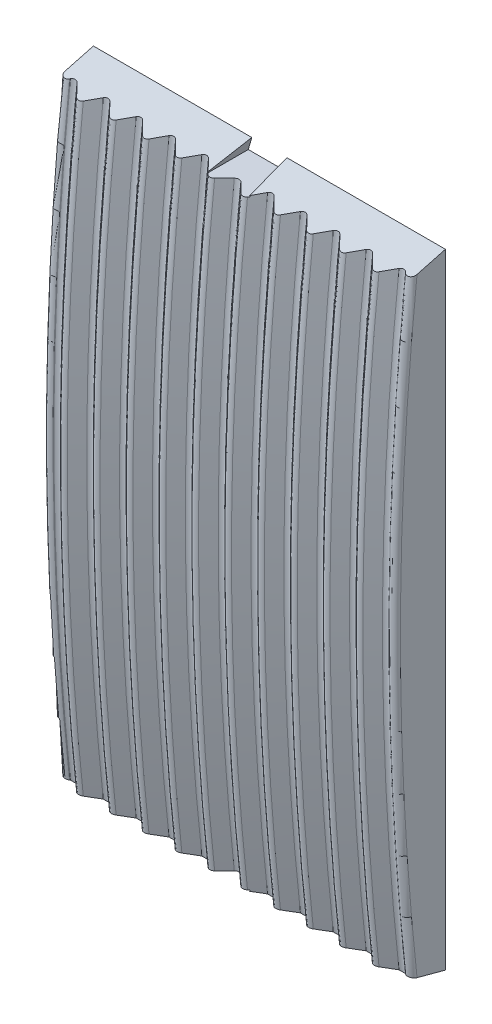
from build123d import *

# Parameters (mm, degrees)
BOSS_EXTRUDE1_DEPTH      = 375
CUT_EXTRUDE1_DEPTH       = 750
LPATTERN1_COUNT          = 6
LPATTERN1_PITCH          = 70
LPATTERN2_COUNT          = 6
LPATTERN2_PITCH          = 70
FILLET1_R                = 10
SKETCH6_W                = 315
SKETCH6_H                = 250
CUT_EXTRUDE2_DEPTH       = 60
CUT_EXTRUDE3_DEPTH       = 335
BOSS_EXTRUDE2_REACH      = 775.751
BOSS_EXTRUDE2_END_RADIUS = 5930
SKETCH8_W                = 40
SKETCH8_H                = 170
SKETCH8_W_2              = 35
SKETCH8_H_2              = 250


with BuildPart() as part:
    # Sketch2 → Boss-Extrude1 (new, symmetric)
    with BuildSketch(Plane(origin=(0, 0, 0), x_dir=(0, 0, -1), z_dir=(1, 0, 0))):
        with BuildLine():
            Line((130, -665), (130, 665))
            Line((130, 665), (34.157984961, 639.319209469))
            ThreePointArc((34.157984961, 639.319209469), (0, 0), (34.157984961, -639.319209469))
            Line((34.157984961, -639.319209469), (130, -665))
        make_face()
    extrude(amount=BOSS_EXTRUDE1_DEPTH, both=True)

    # Sketch3 → Cut-Extrude1 (cut)
    with BuildSketch(Plane(origin=(0, 0, -130), x_dir=(-1, 0, 0), z_dir=(0, 0, -1))):
        Polygon((-37.5, 665), (-45, 639), (45, 639), (37.5, 665), align=None)
    cut_extrude1 = extrude(amount=-CUT_EXTRUDE1_DEPTH, mode=Mode.SUBTRACT)

    # Mirror1: Cut-Extrude1 across plane
    add(cut_extrude1.mirror(Plane.ZX), mode=Mode.SUBTRACT)

    # Cut-Sweep1: sweep along a path in Sketch4
    with BuildLine(Plane(origin=(0, 0, 0), x_dir=(0, 0, -1), z_dir=(1, 0, 0))) as cut_sweep1_path:
        ThreePointArc((36.96595683, 665), (0, 0), (36.96595683, -665))
    # Sketch5 → Cut-Sweep1 (sweep, cut)
    with BuildSketch(Plane(origin=(0, 0, 0), x_dir=(1, 0, 0), z_dir=(0, 1, 0))):
        Polygon((0, 35), (-35, 0), (35, 0), align=None)
    cut_sweep1 = sweep(path=cut_sweep1_path.line, mode=Mode.SUBTRACT)

    # LPattern1: Cut-Sweep1 ×6
    with Locations(*[(-i * LPATTERN1_PITCH, 0, 0) for i in range(1, LPATTERN1_COUNT)]):
        add(cut_sweep1, mode=Mode.SUBTRACT)

    # LPattern2: Cut-Sweep1 ×6
    with Locations(*[(i * LPATTERN2_PITCH, 0, 0) for i in range(1, LPATTERN2_COUNT)]):
        add(cut_sweep1, mode=Mode.SUBTRACT)

    # Fillet1
    fillet1_edges = [part.edges().sort_by_distance(p)[0] for p in [
        (-350, 0, -35),
        (-375, 0, -10),
        (140, 0, -35),
        (210, 0, -35),
        (280, 0, -35),
        (350, 0, -35),
        (375, 0, -10),
        (315, 0, 0),
        (245, 0, 0),
        (175, 0, 0),
        (70, 0, -35),
        (0, 0, -35),
        (105, 0, 0),
        (35, 0, 0),
        (-35, 0, 0),
        (-70, 0, -35),
        (-105, 0, 0),
        (-140, 0, -35),
        (-175, 0, 0),
        (-210, 0, -35),
        (-245, 0, 0),
        (-280, 0, -35),
        (-315, 0, 0),
    ]]
    fillet(fillet1_edges, radius=FILLET1_R)

    # Sketch6 → Cut-Extrude2 (cut)
    with BuildSketch(Plane(origin=(0, 0, -130), x_dir=(-1, 0, 0), z_dir=(0, 0, -1))):
        with Locations((177.5, 0)):
            Rectangle(SKETCH6_W, SKETCH6_H)
        with Locations((-177.5, 0)):
            Rectangle(SKETCH6_W, SKETCH6_H)
    extrude(amount=-CUT_EXTRUDE2_DEPTH, mode=Mode.SUBTRACT)

    # Sketch7 → Cut-Extrude3 (cut, symmetric)
    with BuildSketch(Plane(origin=(0, 0, 0), x_dir=(0, 0, -1), z_dir=(1, 0, 0))):
        with BuildLine():
            Line((130, 625), (130, 455))
            Line((130, 455), (87.481501086, 455))
            ThreePointArc((87.481501086, 455), (94.643145913, 540.055947001), (103.028319552, 625))
            Line((103.028319552, 625), (130, 625))
        make_face()
        with BuildLine():
            Line((130, 415), (130, 165))
            Line((130, 165), (72.295975675, 165))
            ThreePointArc((72.295975675, 165), (77.098470758, 290.064604699), (84.539324786, 415))
            Line((84.539324786, 415), (130, 415))
        make_face()
    cut_extrude3 = extrude(amount=CUT_EXTRUDE3_DEPTH, both=True, mode=Mode.SUBTRACT)

    # Boss-Extrude2: up to this cylinder (the profile starts inside it)
    boss_extrude2_end = Plane(origin=(0, 0, -6000), z_dir=(1, 0, 0)) * Cylinder(BOSS_EXTRUDE2_END_RADIUS, 13647.502, mode=Mode.PRIVATE)
    # Sketch8 → Boss-Extrude2 (add, up to the surface)
    with BuildSketch(Plane(origin=(0, 0, -130), x_dir=(-1, 0, 0), z_dir=(0, 0, -1)), mode=Mode.PRIVATE) as boss_extrude2_sk1:
        with Locations((0, 540)):
            Rectangle(SKETCH8_W, SKETCH8_H)
    boss_extrude2_tool1 = extrude(boss_extrude2_sk1.sketch, amount=-BOSS_EXTRUDE2_REACH, mode=Mode.PRIVATE) & boss_extrude2_end
    # Sketch8 → Boss-Extrude2 (add, up to the surface)
    with BuildSketch(Plane(origin=(0, 0, -130), x_dir=(-1, 0, 0), z_dir=(0, 0, -1)), mode=Mode.PRIVATE) as boss_extrude2_sk2:
        with Locations((-117.5, 290)):
            Rectangle(SKETCH8_W_2, SKETCH8_H_2)
    boss_extrude2_tool2 = extrude(boss_extrude2_sk2.sketch, amount=-BOSS_EXTRUDE2_REACH, mode=Mode.PRIVATE) & boss_extrude2_end
    # Sketch8 → Boss-Extrude2 (add, up to the surface)
    with BuildSketch(Plane(origin=(0, 0, -130), x_dir=(-1, 0, 0), z_dir=(0, 0, -1)), mode=Mode.PRIVATE) as boss_extrude2_sk3:
        with Locations((117.5, 290)):
            Rectangle(SKETCH8_W_2, SKETCH8_H_2)
    boss_extrude2_tool3 = extrude(boss_extrude2_sk3.sketch, amount=-BOSS_EXTRUDE2_REACH, mode=Mode.PRIVATE) & boss_extrude2_end
    boss_extrude2 = boss_extrude2_tool1.solids().sort_by_distance((0, 540, -130))[0] + boss_extrude2_tool2.solids().sort_by_distance((117.5, 290, -130))[0] + boss_extrude2_tool3.solids().sort_by_distance((-117.5, 290, -130))[0]
    add(boss_extrude2)

    # Mirror3: Cut-Extrude3, Boss-Extrude2 across plane
    add(cut_extrude3.mirror(Plane.ZX), mode=Mode.SUBTRACT)
    add(boss_extrude2.mirror(Plane.ZX))


solid = part.part
